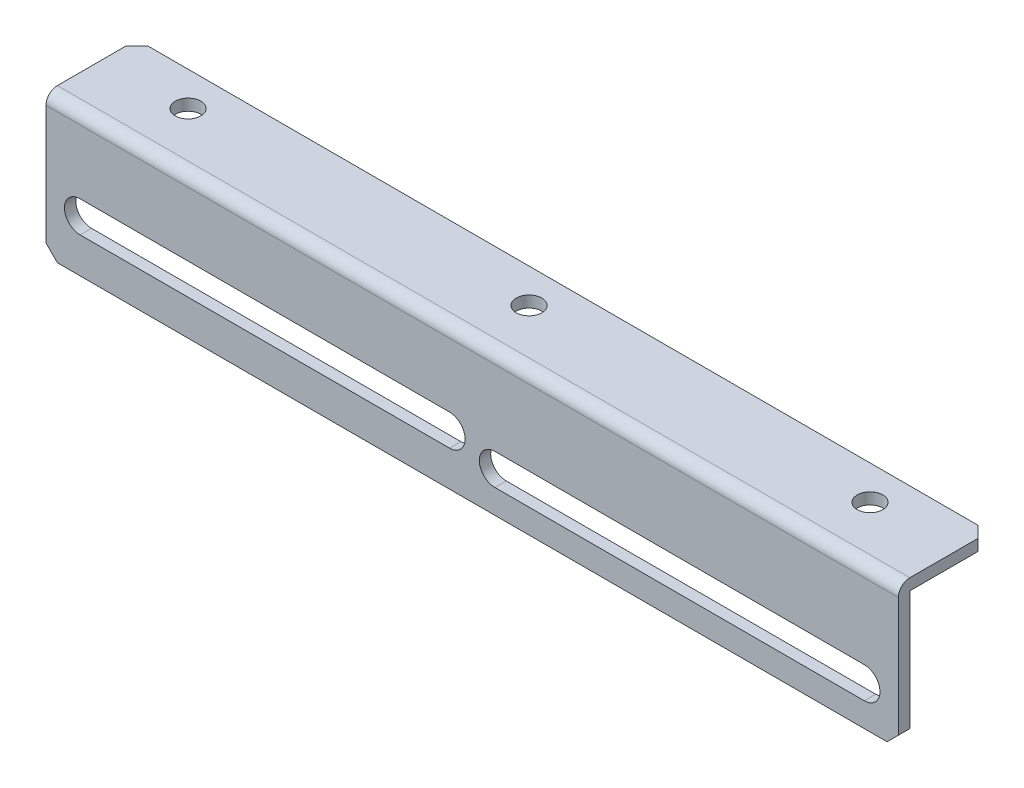
SolidWorks part; units mm, degrees
ref_plane "Front Plane" through (0, 0, 0) normal (0, 0, 1) x (1, 0, 0)
ref_plane "Top Plane" through (0, 0, 0) normal (0, 1, 0) x (1, 0, 0)
ref_plane "Right Plane" through (0, 0, 0) normal (1, 0, 0) x (0, 0, -1)
ref_plane "Plane 4" through (0, 0, 0) normal (0, 0, -1) x (-1, 0, 0)
sketch "Sketch 1" plane through (0, 0, 0) normal (0, 0, -1) x (-1, 0, 0)
  line L0 (75, 12.5) -> (-75, 12.5)
  line L1 (-75, 12.5) -> (-75, -12.5)
  line L2 (-75, -12.5) -> (75, -12.5)
  line L3 (75, -12.5) -> (75, 12.5)
extrude "Boss-Extrude 1" add sketch "Sketch 1" against normal blind 18
sketch "Sketch 2" plane through (-75, 0, 0) normal (-1, 0, 0) x (0, 0, 1)
  line L0 (16, -12.5) -> (16, 10.5)
  line L1 (16, 10.5) -> (0, 10.5)
  line L2 (0, 10.5) -> (0, -12.5)
  line L3 (0, -12.5) -> (16, -12.5)
extrude "Cut-Extrude 1" cut sketch "Sketch 2" against normal through all
sketch "Sketch 3" plane through (0, 0, 16) normal (0, 0, -1) x (-1, 0, 0)
  line L0 (-4, -2.75) -> (-69, -2.75)
  line L1 (-69, -8.25) -> (-4, -8.25)
  line L2 (75, 12.5) -> (-75, 12.5) construction
  arc A0 (-69, -2.75) -> (-69, -8.25) centre (-69, -5.5) ccw
  arc A1 (-4, -8.25) -> (-4, -2.75) centre (-4, -5.5) ccw
  dimension "D1" = 18
extrude "Cut-Extrude 2" cut sketch "Sketch 3" against normal through all
sketch "Sketch 4" plane through (0, 0, 18) normal (0, 0, 1) x (1, 0, 0)
  line L0 (-69, -6.25) -> (-4, -6.25)
  line L1 (-4, -0.75) -> (-69, -0.75)
  line L2 (-75, 12.5) -> (75, 12.5) construction
  arc A0 (-4, -6.25) -> (-4, -0.75) centre (-4, -3.5) ccw
  arc A1 (-69, -0.75) -> (-69, -6.25) centre (-69, -3.5) ccw
  dimension "D1" = 16
extrude "Cut-Extrude 3" cut sketch "Sketch 4" against normal through all
hole_wizard "Ø4.5 (4.5) Hole 1" positions "Sketch 6" profile "Sketch 5" hole size "Ø4.5" standard "GB"
sketch "Sketch 6" plane through (0, 12.5, 0) normal (0, 1, 0) x (-1, 0, 0)
  line L0 (75, 18) -> (-75, 18) construction
  point P0 (-60, 8)
  dimension "D1" = 10
sketch "Sketch 5" plane through (60, 12.5, 8) normal (1, 0, 0) x (0, 0, 1)
  line L0 (0, 0) -> (0, 16.3519)
  line L1 (0, 16.3519) -> (2.25, 15)
  line L2 (2.25, 15) -> (2.25, 0)
  line L5 (2.25, 0) -> (0, 0)
  line L10 (0, 16.3519) -> (-2.25, 15) construction
  line L11 (0, -6.35) -> (0, 107.95) construction
  dimension "鑽孔直徑" = 4.5
  dimension "鑽孔深度" = 15
  dimension "導頭角度" = 118
hole_wizard "Ø4.5 (4.5) Hole 3" positions "Sketch 8" profile "Sketch 7" hole size "Ø4.5" standard "GB"
sketch "Sketch 8" plane through (0, 12.5, 0) normal (0, 1, 0) x (-1, 0, 0)
  line L0 (75, 18) -> (-75, 18) construction
  point P0 (60, 8)
  dimension "D1" = 10
sketch "Sketch 7" plane through (-60, 12.5, 8) normal (1, 0, 0) x (0, 0, 1)
  line L0 (0, 0) -> (0, 16.3519)
  line L1 (0, 16.3519) -> (2.25, 15)
  line L2 (2.25, 15) -> (2.25, 0)
  line L5 (2.25, 0) -> (0, 0)
  line L10 (0, 16.3519) -> (-2.25, 15) construction
  line L11 (0, -6.35) -> (0, 107.95) construction
  dimension "鑽孔直徑" = 4.5
  dimension "鑽孔深度" = 15
  dimension "導頭角度" = 118
hole_wizard "Ø4.5 (4.5) Hole 2" positions "Sketch 10" profile "Sketch 9" hole size "Ø4.5" standard "GB"
sketch "Sketch 10" plane through (0, 12.5, 0) normal (0, 1, 0) x (-1, 0, 0)
  line L0 (75, 18) -> (-75, 18) construction
  point P0 (0, 8)
  dimension "D1" = 10
sketch "Sketch 9" plane through (0, 12.5, 8) normal (1, 0, 0) x (0, 0, 1)
  line L0 (0, 0) -> (0, 16.3519)
  line L1 (0, 16.3519) -> (2.25, 15)
  line L2 (2.25, 15) -> (2.25, 0)
  line L5 (2.25, 0) -> (0, 0)
  line L10 (0, 16.3519) -> (-2.25, 15) construction
  line L11 (0, -6.35) -> (0, 107.95) construction
  dimension "鑽孔直徑" = 4.5
  dimension "鑽孔深度" = 15
  dimension "導頭角度" = 118
chamfer "Chamfer 1" distance 2 angle 45 1 edges at (75, -12.5, 17)
chamfer "Chamfer 3" distance 2 angle 45 1 edges at (-75, -12.5, 17)
fillet "Fillet 1" radius 2 1 edges at (0, 12.5, 18)
sketch "Sketch 11" plane through (0, 12.5, 0) normal (0, 1, 0) x (1, 0, 0)
  line L0 (-75, -16) -> (-75, 0) construction
  line L1 (75, 0) -> (-75, 0)
  line L2 (75, 0) -> (75, -2)
  line L3 (75, -2) -> (-75, -2)
  line L4 (-75, 0) -> (-75, -2)
  dimension "D1" = 2
extrude "Cut-Extrude 4" cut sketch "Sketch 11" against normal blind 10
chamfer "Chamfer 4" distance 2 angle 45 2 edges at (75, 11.5, 2) (-75, 11.5, 2)
